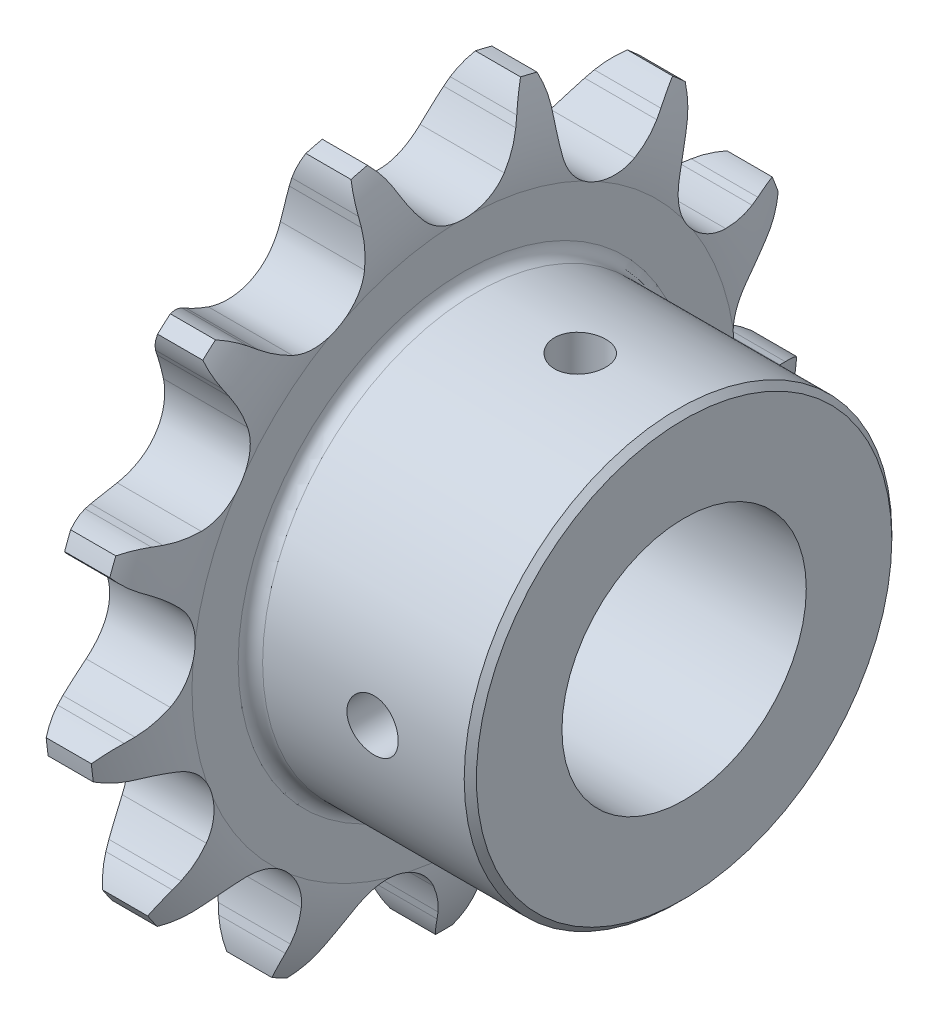
from build123d import *

# Parameters (mm, degrees)
CUT_EXTRUDE_1_DEPTH      = 4.638656443
PATTERN_CIRCULAR_1_COUNT = 13
SKETCH_3_R               = 17.5
SKETCH_3_R_2             = 10
EXTRUDE_1_DEPTH          = 18
FILLET_1_R               = 1
CHAMFER_1_SIZE           = 0.5
HOLE_WIZARD_M5_1_D       = 4.2
HOLE_WIZARD_M5_1_DEPTH   = 12.4
HOLE_WIZARD_M5_1_TIP     = 1.2618073
HOLE_WIZARD_M5_2_D       = 4.2
HOLE_WIZARD_M5_2_DEPTH   = 12.4
HOLE_WIZARD_M5_2_TIP     = 1.2618073


with BuildPart() as part:
    # 草图1 → 旋转1 (revolve)
    with BuildSketch(Plane.XY, mode=Mode.PRIVATE) as revolve_1_sk:
        with BuildLine():
            Line((-3.5, 10), (-3.5, 22.278992327))
            ThreePointArc((-3.5, 22.278992327), (-3.141151912, 25.754128127), (-1.849, 29))
            Line((-1.849, 29), (1.849, 29))
            ThreePointArc((1.849, 29), (3.141151912, 25.754128127), (3.5, 22.278992327))
            Line((3.5, 22.278992327), (3.5, 10))
            Line((3.5, 10), (-3.5, 10))
        make_face()
    revolve(revolve_1_sk.sketch.rotate(Axis((-6.35, 0, 0), (1, 0, 0)), 90), axis=Axis((-6.35, 0, 0), (1, 0, 0)))

    # 草图2 → 切除-拉伸1 (cut, symmetric)
    with BuildSketch(Plane(origin=(0, 0, 0), x_dir=(0, 0, -1), z_dir=(1, 0, 0))):
        with BuildLine():
            Line((4.769475288, 26.007478281), (5.07686592, 26.639875941))
            ThreePointArc((5.07686592, 26.639875941), (5.601425484, 27.526379428), (6.263467786, 28.31552527))
            ThreePointArc((6.263467786, 28.31552527), (0, 29), (-6.263467786, 28.31552527))
            ThreePointArc((-6.263467786, 28.31552527), (-5.601425484, 27.526379428), (-5.07686592, 26.639875941))
            Line((-5.07686592, 26.639875941), (-4.769475288, 26.007478281))
            ThreePointArc((-4.769475288, 26.007478281), (-4.11784871, 24.848481966), (-3.332711591, 23.775425883))
            ThreePointArc((-3.332711591, 23.775425883), (0, 22.207717327), (3.332711591, 23.775425883))
            ThreePointArc((3.332711591, 23.775425883), (4.11784871, 24.848481966), (4.769475288, 26.007478281))
        make_face()
    cut_extrude_1 = extrude(amount=CUT_EXTRUDE_1_DEPTH, both=True, mode=Mode.SUBTRACT)

    # 阵列(圆周)1: 切除-拉伸1 ×13 about axis
    pattern_circular_1_axis = Axis((0, 0, 0), (1, 0, 0))
    for i in range(1, PATTERN_CIRCULAR_1_COUNT):
        add(cut_extrude_1.rotate(pattern_circular_1_axis, i * 360 / PATTERN_CIRCULAR_1_COUNT), mode=Mode.SUBTRACT)

    # 草图3 → 凸台-拉伸1 (add)
    with BuildSketch(Plane(origin=(3.5, 0, 0), x_dir=(0, 0, -1), z_dir=(1, 0, 0))):
        with Locations(Location((0, 0, 0), (0, 0, 180))):
            Circle(SKETCH_3_R)
        with Locations(Location((0, 0, 0), (0, 0, 180))):
            Circle(SKETCH_3_R_2, mode=Mode.SUBTRACT)
    extrude(amount=EXTRUDE_1_DEPTH)

    # 圆角1
    fillet_1_edges = [part.edges().sort_by_distance(p)[0] for p in [
        (3.5, 0, -17.5),
    ]]
    fillet(fillet_1_edges, radius=FILLET_1_R)

    # 倒角1
    chamfer_1_edges = [part.edges().sort_by_distance(p)[0] for p in [
        (21.5, 0, -17.5),
    ]]
    chamfer(chamfer_1_edges, length=CHAMFER_1_SIZE)

    # M5 螺纹孔1
    with Locations(Plane(origin=(0, 17.5, 0), x_dir=(1, 0, 0), z_dir=(0, 1, 0))):
        with Locations((13, 0)):
            Hole(HOLE_WIZARD_M5_1_D / 2, depth=HOLE_WIZARD_M5_1_DEPTH)
            with Locations((0, 0, -(HOLE_WIZARD_M5_1_DEPTH + HOLE_WIZARD_M5_1_TIP / 2))):  # 118° drill point
                Cone(0, HOLE_WIZARD_M5_1_D / 2, HOLE_WIZARD_M5_1_TIP, mode=Mode.SUBTRACT)

    # M5 螺纹孔2
    with Locations(Plane.XY.offset(17.5)):
        with Locations((13.5, 0)):
            Hole(HOLE_WIZARD_M5_2_D / 2, depth=HOLE_WIZARD_M5_2_DEPTH)
            with Locations((0, 0, -(HOLE_WIZARD_M5_2_DEPTH + HOLE_WIZARD_M5_2_TIP / 2))):  # 118° drill point
                Cone(0, HOLE_WIZARD_M5_2_D / 2, HOLE_WIZARD_M5_2_TIP, mode=Mode.SUBTRACT)


solid = part.part
